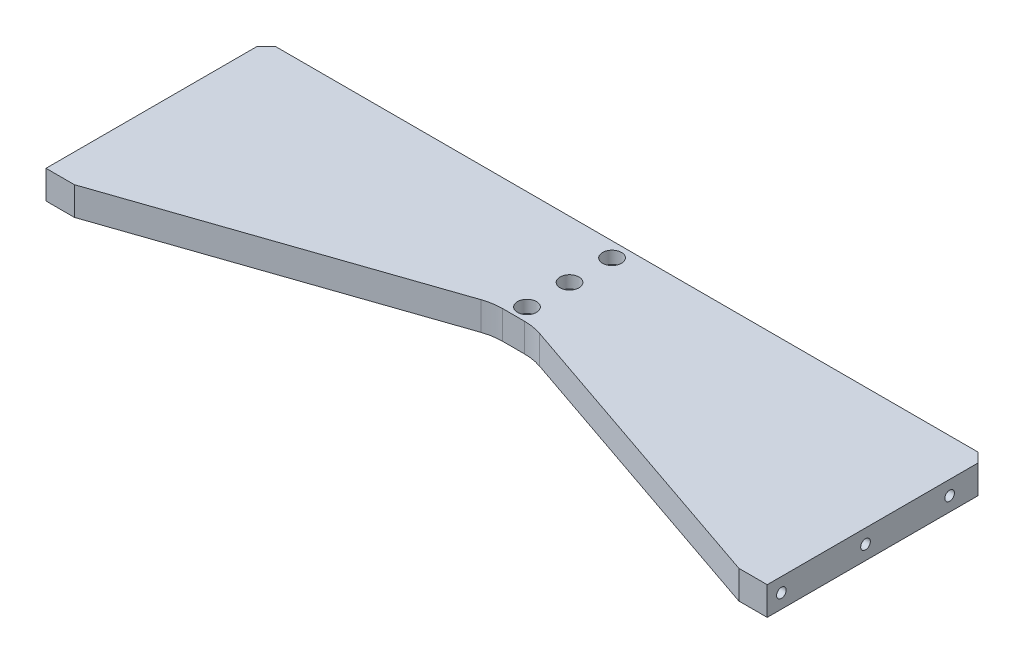
from build123d import *

# Parameters (mm, degrees)
SKETCH_1_W                = 763
SKETCH_1_H                = 233
EXTRUDE_1_DEPTH           = 30
CHAMFER_1_SIZE            = 10
CUT_EXTRUDE_1_DEPTH       = 401.018124589
CUT_EXTRUDE_1_DEPTH_BACK  = 30
FILLET_1_R                = 60
HOLE_WIZARD_1_D           = 13.5
HOLE_WIZARD_1_CBORE_D     = 20
HOLE_WIZARD_1_CBORE_DEPTH = 13
HOLE_WIZARD_M12_1_D       = 10.2
HOLE_WIZARD_M12_1_DEPTH   = 29.25
HOLE_WIZARD_M12_1_TIP     = 3.064389157
HOLE_WIZARD_M12_2_D       = 10.2
HOLE_WIZARD_M12_2_DEPTH   = 29.25
HOLE_WIZARD_M12_2_TIP     = 3.064389157
HOLE_WIZARD_M12_3_D       = 10.2
HOLE_WIZARD_M12_3_DEPTH   = 29.25
HOLE_WIZARD_M12_3_TIP     = 3.064389157


with BuildPart() as part:
    # 草图1 → 凸台-拉伸1 (new body)
    with BuildSketch(Plane(origin=(0, 0, 0), x_dir=(1, 0, 0), z_dir=(0, 1, 0))):
        Rectangle(SKETCH_1_W, SKETCH_1_H)
    extrude(amount=EXTRUDE_1_DEPTH)

    # 倒角1
    chamfer_1_edges = [part.edges().sort_by_distance(p)[0] for p in [
        (-381.5, 15, -116.5),
        (381.5, 15, -116.5),
    ]]
    chamfer(chamfer_1_edges, length=CHAMFER_1_SIZE)

    # 草图2 → 切除-拉伸1 (cut, two sides: drawn at the far end of the back side and taken through both)
    with BuildSketch(Plane(origin=(0, 30, 0), x_dir=(1, 0, 0), z_dir=(0, 1, 0)).offset(-CUT_EXTRUDE_1_DEPTH_BACK)):
        Polygon((-1816.285660926, -618.078120257), (-351.5, -116.5), (-21.5, -3.5), (21.5, -3.5), (351.5, -116.5), (1816.285660926, -618.078120257), (1816.285660926, -3714.642437803), (-1816.285660926, -3714.642437803), align=None)
    extrude(amount=CUT_EXTRUDE_1_DEPTH + CUT_EXTRUDE_1_DEPTH_BACK, mode=Mode.SUBTRACT)

    # 圆角1
    fillet_1_edges = [part.edges().sort_by_distance(p)[0] for p in [
        (21.5, 15, 3.5),
        (-21.5, 15, 3.5),
    ]]
    fillet(fillet_1_edges, radius=FILLET_1_R)

    # 打孔尺寸(%根据)内六角圆柱头螺钉的类型1 (through all)
    with Locations(Plane(origin=(0, 30, 0), x_dir=(1, 0, 0), z_dir=(0, 1, 0))):
        with Locations((0, 100.862096352), (0, 55.862096352), (0, 10.862096352)):
            CounterBoreHole(HOLE_WIZARD_1_D / 2, HOLE_WIZARD_1_CBORE_D / 2, HOLE_WIZARD_1_CBORE_DEPTH)

    # M12 螺纹孔1
    with Locations(Plane(origin=(0, 0, -116.5), x_dir=(-1, 0, 0), z_dir=(0, 0, -1))):
        with Locations((351.5, 15), (251.071428571, 15), (150.642857143, 15), (50.214285714, 15), (-50.214285714, 15), (-150.642857143, 15), (-251.071428571, 15), (-351.5, 15)):
            Hole(HOLE_WIZARD_M12_1_D / 2, depth=HOLE_WIZARD_M12_1_DEPTH)
            with Locations((0, 0, -(HOLE_WIZARD_M12_1_DEPTH + HOLE_WIZARD_M12_1_TIP / 2))):  # 118° drill point
                Cone(0, HOLE_WIZARD_M12_1_D / 2, HOLE_WIZARD_M12_1_TIP, mode=Mode.SUBTRACT)

    # M12 螺纹孔2
    with Locations(Plane(origin=(381.5, 0, 0), x_dir=(0, 0, -1), z_dir=(1, 0, 0))):
        with Locations((76.5, 15), (-12.5, 15), (-101.5, 15)):
            Hole(HOLE_WIZARD_M12_2_D / 2, depth=HOLE_WIZARD_M12_2_DEPTH)
            with Locations((0, 0, -(HOLE_WIZARD_M12_2_DEPTH + HOLE_WIZARD_M12_2_TIP / 2))):  # 118° drill point
                Cone(0, HOLE_WIZARD_M12_2_D / 2, HOLE_WIZARD_M12_2_TIP, mode=Mode.SUBTRACT)

    # M12 螺纹孔3
    with Locations(Plane.ZY.offset(381.5)):
        with Locations((-76.5, 15), (12.5, 15), (101.5, 15)):
            Hole(HOLE_WIZARD_M12_3_D / 2, depth=HOLE_WIZARD_M12_3_DEPTH)
            with Locations((0, 0, -(HOLE_WIZARD_M12_3_DEPTH + HOLE_WIZARD_M12_3_TIP / 2))):  # 118° drill point
                Cone(0, HOLE_WIZARD_M12_3_D / 2, HOLE_WIZARD_M12_3_TIP, mode=Mode.SUBTRACT)


solid = part.part
